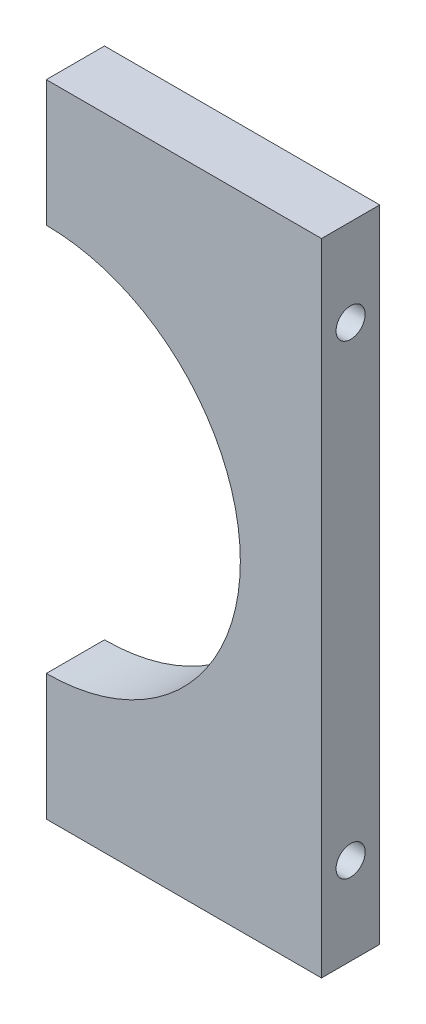
from build123d import *

# Parameters (mm, degrees)
BOSS_EXTRUDE1_DEPTH = 3
SKETCH3_R           = 0.75
CUT_EXTRUDE1_DEPTH  = 31.209452006


with BuildPart() as part:
    # Sketch2 → Boss-Extrude1 (new body)
    with BuildSketch(Plane.XY):
        with BuildLine():
            Line((16.5, -26.504131531), (30.682454029, -26.504131531))
            Line((30.682454029, -26.504131531), (30.682454029, 6.495868469))
            Line((30.682454029, 6.495868469), (16.5, 6.495868469))
            Line((16.5, 6.495868469), (16.5, -0.004131531))
            ThreePointArc((16.5, -0.004131531), (26.5, -10.004131531), (16.5, -20.004131531))
            Line((16.5, -20.004131531), (16.5, -26.504131531))
        make_face()
    extrude(amount=-BOSS_EXTRUDE1_DEPTH)

    # Sketch3 → Cut-Extrude1 (cut, through all)
    with BuildSketch(Plane(origin=(30.682454029, 0, 0), x_dir=(0, 0, -1), z_dir=(1, 0, 0))):
        with Locations((1.5, -22.004131531)):
            Circle(SKETCH3_R)
        with Locations(Location((1.5, 1.995868469, 0), (0, 0, 180))):
            Circle(SKETCH3_R)
    extrude(amount=-CUT_EXTRUDE1_DEPTH, mode=Mode.SUBTRACT)


solid = part.part
